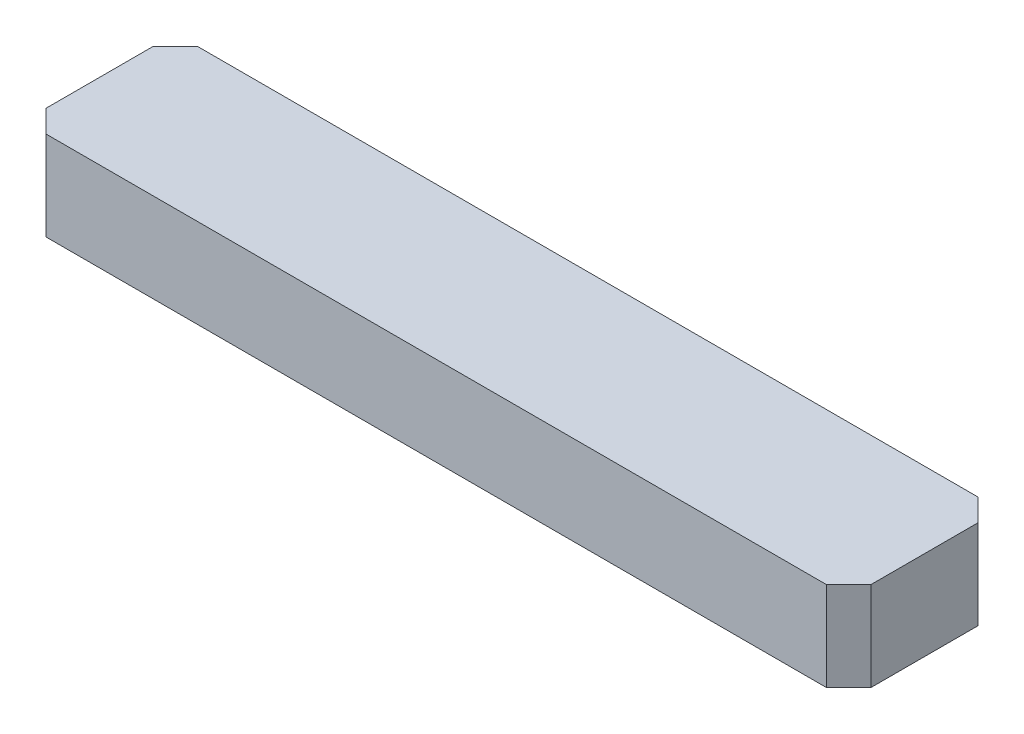
SolidWorks part; units mm, degrees
ref_plane "Front Plane" through (0, 0, 0) normal (0, 0, 1) x (1, 0, 0)
ref_plane "Top Plane" through (0, 0, 0) normal (0, 1, 0) x (1, 0, 0)
ref_plane "Right Plane" through (0, 0, 0) normal (1, 0, 0) x (0, 0, -1)
sketch "Sketch1" plane through (0, 0, 0) normal (0, 1, 0) x (1, 0, 0)
  line L1 (-18.5, 3.4) -> (18.5, 3.4)
  line L2 (-18.5, 3.4) -> (-18.5, -3.4)
  line L3 (-18.5, -3.4) -> (18.5, -3.4)
  line L4 (18.5, 3.4) -> (18.5, -3.4)
  line L5 (-18.5, 3.4) -> (18.5, -3.4) construction
  line L6 (-18.5, -3.4) -> (18.5, 3.4) construction
  point P0 (0, 0)
  dimension "D1" = 6.8
  dimension "D2" = 37
extrude "Boss-Extrude1" add sketch "Sketch1" along normal mid plane 4
chamfer "Chamfer1" distance 1 angle 45 4 edges at (-18.5, 0, -3.4) (-18.5, 0, 3.4) (18.5, 0, -3.4) (18.5, 0, 3.4)
